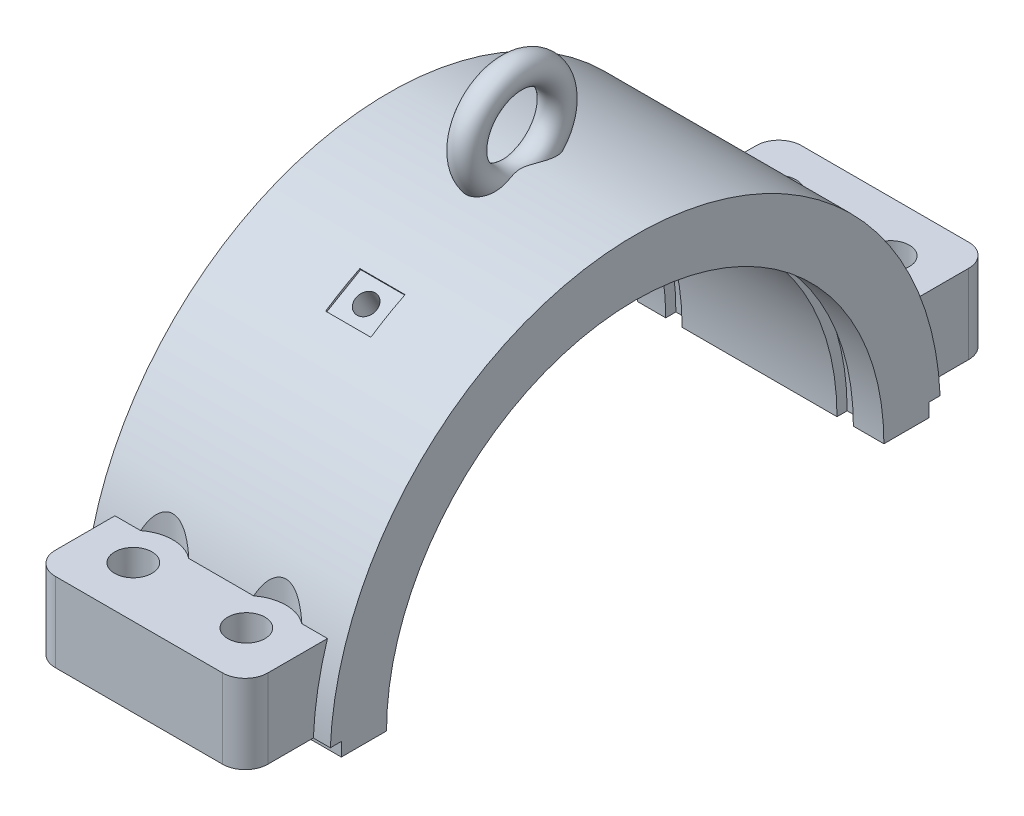
from build123d import *

# Parameters (mm, degrees)
BOSS_EXTRUDE2_DEPTH    = 109
BOSS_EXTRUDE3_DEPTH    = 94
SKETCH5_R              = 16.5
CUT_EXTRUDE1_DEPTH     = 396.126562003
CUT_EXTRUDE2_START     = 82
SKETCH6_R              = 35
CUT_EXTRUDE2_DEPTH     = 19.98039
SKETCH7_W              = 39.278789695
SKETCH7_H              = 17.735547429
CUT_EXTRUDE3_DEPTH     = 441.092035915
FILLET1_R              = 20
FILLET1_OF_MIRROR1_R   = 20
SKETCH8_W              = 14.5
SKETCH8_H              = 9
SKETCH9_R              = 12.5
CUT_EXTRUDE4_START     = 5
CUT_EXTRUDE4_DEPTH     = 20
M20X1_5_TAPPED_HOLE1_D = 18.5


with BuildPart() as part:
    # Sketch1 → Boss-Extrude2 (new, symmetric)
    with BuildSketch(Plane(origin=(0, 0, 0), x_dir=(0, 0, -1), z_dir=(1, 0, 0))):
        with BuildLine():
            Line((-270, 0), (-220, 0))
            ThreePointArc((-220, 0), (0, 220), (220, 0))
            Line((220, 0), (270, 0))
            ThreePointArc((270, 0), (0, 270), (-270, 0))
        make_face()
    extrude(amount=BOSS_EXTRUDE2_DEPTH, both=True)

    # Sketch4 → Boss-Extrude3 (add, symmetric)
    with BuildSketch(Plane(origin=(0, 0, 0), x_dir=(0, 0, -1), z_dir=(1, 0, 0))):
        with BuildLine():
            Line((-330, 12), (-269.733201516, 12))
            ThreePointArc((-269.733201516, 12), (-265.804483526, 47.41283094), (-257.246963053, 82))
            Line((-257.246963053, 82), (-330, 82))
            Line((-330, 82), (-330, 12))
        make_face()
    boss_extrude3 = extrude(amount=BOSS_EXTRUDE3_DEPTH, both=True)

    # Sketch5 → Cut-Extrude1 (cut, symmetric)
    with BuildSketch(Plane(origin=(0, 82, 0), x_dir=(1, 0, 0), z_dir=(0, 1, 0))):
        with Locations(Location((50, -285, 0), (0, 0, 65.380022671))):
            Circle(SKETCH5_R)
        with Locations(Location((-50, -285, 0), (0, 0, 65.380022671))):
            Circle(SKETCH5_R)
    cut_extrude1 = extrude(amount=CUT_EXTRUDE1_DEPTH, both=True, mode=Mode.SUBTRACT)

    # Sketch6 → Cut-Extrude2 (cut)
    with BuildSketch(Plane(origin=(0, 0, 0), x_dir=(1, 0, 0), z_dir=(0, 1, 0)).offset(CUT_EXTRUDE2_START)):
        with Locations((-50, -285)):
            Circle(SKETCH6_R)
        with Locations((50, -285)):
            Circle(SKETCH6_R)
    cut_extrude2 = extrude(amount=CUT_EXTRUDE2_DEPTH, mode=Mode.SUBTRACT)

    # Sketch7 → Cut-Extrude3 (cut, symmetric)
    with BuildSketch(Plane(origin=(0, 0, 0), x_dir=(0, 0, -1), z_dir=(1, 0, 0))):
        with Locations((-279.639394848, 3.132226285)):
            Rectangle(SKETCH7_W, SKETCH7_H)
    cut_extrude3 = extrude(amount=CUT_EXTRUDE3_DEPTH, both=True, mode=Mode.SUBTRACT)

    # Fillet1
    fillet1_edges = [part.edges().sort_by_distance(p)[0] for p in [
        (-94, 47, 330),
        (94, 47, 330),
    ]]
    fillet(fillet1_edges, radius=FILLET1_R)

    # Mirror1: Boss-Extrude3, Cut-Extrude1, Cut-Extrude2, Cut-Extrude3 across plane
    add(boss_extrude3.mirror(Plane.XY))
    add(cut_extrude1.mirror(Plane.XY), mode=Mode.SUBTRACT)
    add(cut_extrude2.mirror(Plane.XY), mode=Mode.SUBTRACT)
    add(cut_extrude3.mirror(Plane.XY), mode=Mode.SUBTRACT)

    # Fillet1 of Mirror1
    fillet1_of_mirror1_edges = [part.edges().sort_by_distance(p)[0] for p in [
        (-94, 47, -330),
        (94, 47, -330),
    ]]
    fillet(fillet1_of_mirror1_edges, radius=FILLET1_OF_MIRROR1_R)

    # Sketch8 → Cut-Revolve1 (revolve, cut)
    with BuildSketch(Plane.XY):
        with Locations((-76.75, 224.5)):
            Rectangle(SKETCH8_W, SKETCH8_H)
        with Locations((74.75, 224.5)):
            Rectangle(SKETCH8_W, SKETCH8_H)
    revolve(axis=Axis((0, 0, 0), (1, 0, 0)), mode=Mode.SUBTRACT)

    # Sketch9 → Revolve1 (revolve)
    with BuildSketch(Plane.XY, mode=Mode.PRIVATE) as revolve1_sk:
        with Locations((0, 340)):
            Circle(SKETCH9_R)
    revolve(revolve1_sk.sketch.rotate(Axis((0, 300, 0), (1, 0, 0)), 340.461761532), axis=Axis((0, 300, 0), (1, 0, 0)))

    # Sketch10 → Cut-Extrude4 (cut, symmetric)
    with BuildSketch(Plane(origin=(0, 0, 0), x_dir=(0, 0, -1), z_dir=(1, 0, 0)).offset(CUT_EXTRUDE4_START)):
        Polygon((-149.155444566, 223.344808214), (-118.844555434, 240.844808214), (-120.844555434, 244.308909829), (-151.155444566, 226.808909829), align=None)
    extrude(amount=CUT_EXTRUDE4_DEPTH, both=True, mode=Mode.SUBTRACT)

    # M20x1.5 Tapped Hole1 (through all)
    with Locations(Plane(origin=(5, 232.094808214, 134), x_dir=(0, -0.5, 0.866025403784), z_dir=(0, 0.866025403784, 0.5))):
        with Locations((0, 0)):
            Hole(M20X1_5_TAPPED_HOLE1_D / 2)


solid = part.part
